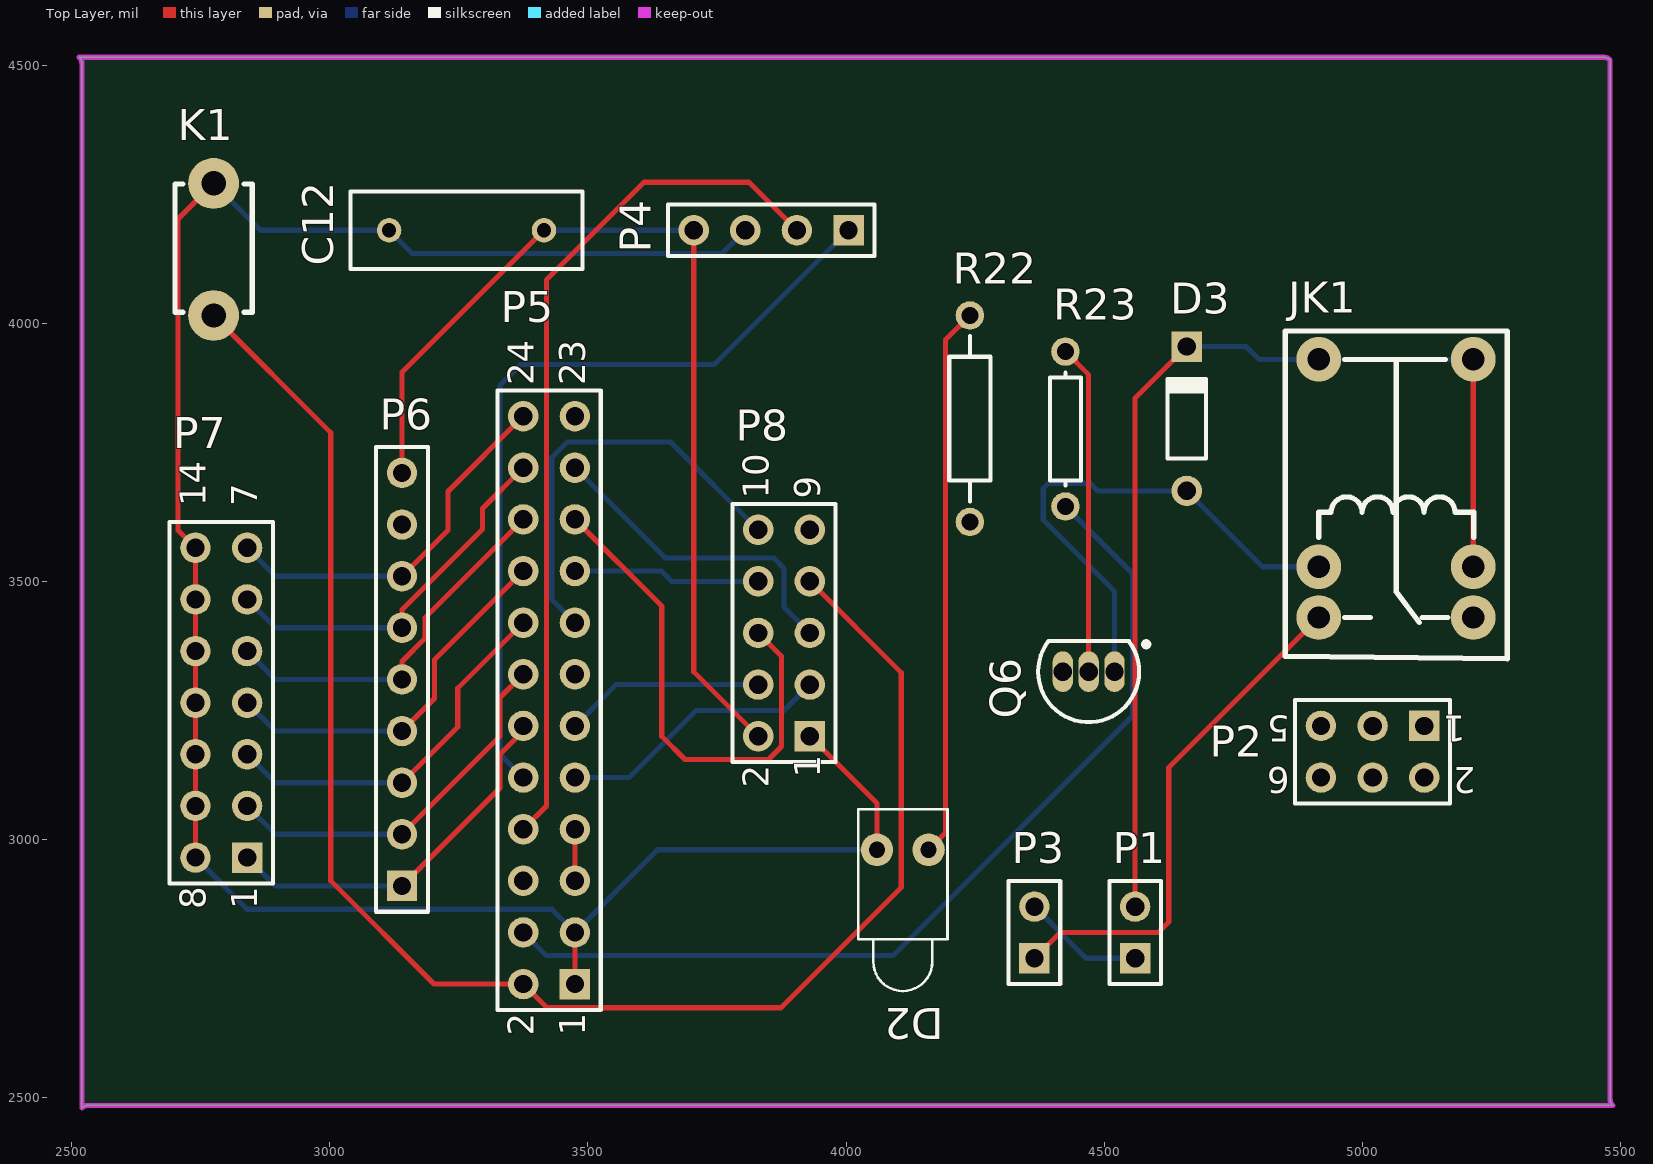
[diagram p0: Top Layer view]
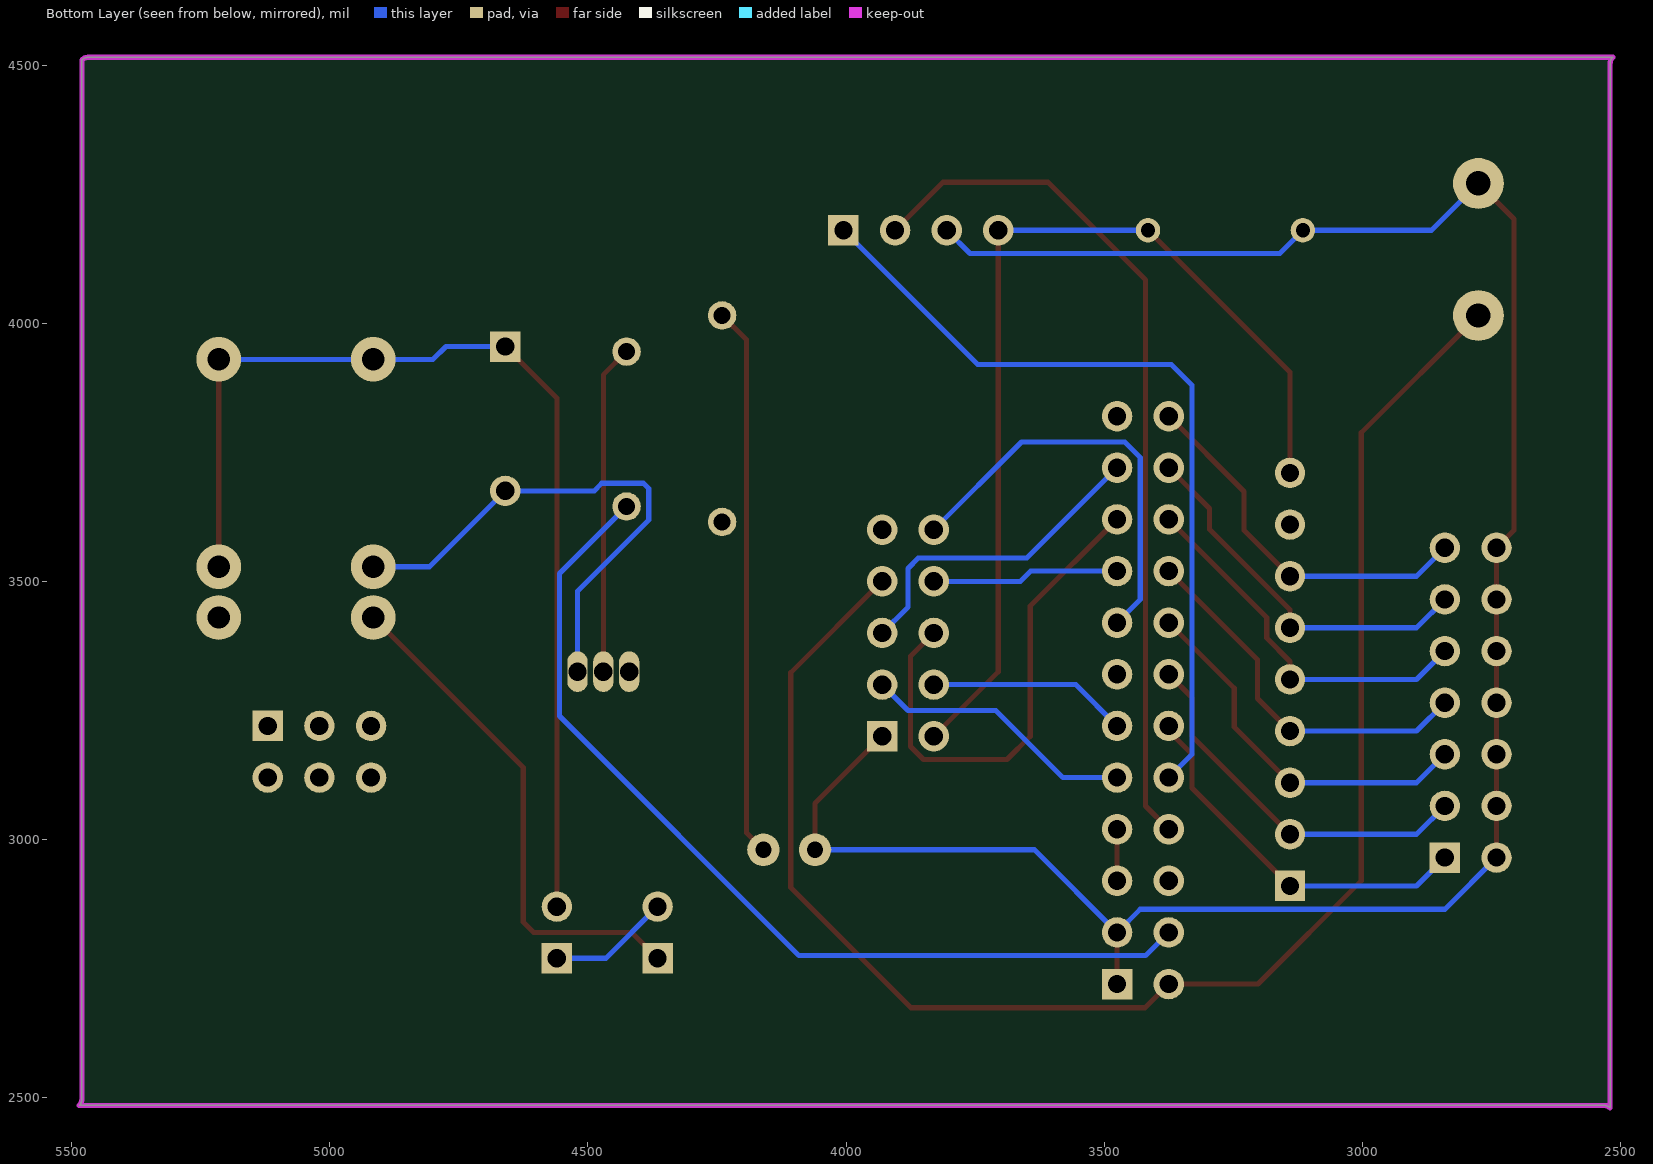
[diagram p1: Bottom Layer view, seen from below]
# Altium PCB MISC80684-5.PcbDoc
Units mil, origin at the board's own origin, x right, y up, seen from the top; angles counter-clockwise.
Board outline 2970 x 2035 mil, 2 copper layers (Top Layer, Bottom Layer); 16 components, 59 nets, 92 pads, 0 vias.

## Layer stack, top to bottom (the 12.6 mil dielectric is the usual default, probably not edited)
Top Solder: solder mask 0.4, Solder Resist, Dk 3.5
Top Layer: signal copper 1.4
Dielectric 1: dielectric 12.6, FR-4, Dk 4.8
Bottom Layer: signal copper 1.4
Bottom Solder: solder mask 0.4, Solder Resist, Dk 3.5

## Board outline
2520,2480 cw(c2532.07,2467.93) 2532.07,2485 5485,2485 cw(c5497.07,2497.07) 5480,2497.07 5480,4510 ccw(c5467.93,4497.93) 5467.93,4515 2515,4515 cw(c2502.93,4502.93) 2520,4502.93

## Design rules (kind name [scope] priority, off if disabled: settings)
Clearance [All] p1: gap=10
PolygonConnect [All] p1: connectstyle=Relief reliefconductorwidth=10 reliefentries=4 polygonreliefangle="90 Angle" airgapwidth=10
RoutingVias [All] p1: holewidth=28 width=50 viastyle="Through Hole" minholewidth=28 minwidth=50 maxholewidth=28 maxwidth=50
SolderMaskExpansion [All] p1: expansion=4
Width [All] p1: maxlimit=10 minlimit=10 preferedwidth=10
30 further rules are at their usual default settings.

## Components (designator, comment, footprint, x,y, rotation, side; value= is the part's Value field where it differs from the comment)
C12 "Cap" RAD-0.3 3265,4180 r180 top
D2 "LED1" LED-1 4110,2980 r270 top
D3 "Diode 1N914" DO-35 4660,3815 r90 top
JK1 "HRS1H-S-DC5V" HRS1H 4915.79,3930 r90 top
K1 "KEY" DIP-3X6X4.3 2775,4015 r90 top
P1 "Header 2" HDR1X2 4560,2770 r90 top
P2 "220V-5V-3.3V" HDR2X3 5120,3220 r180 top
P3 "Header 2" HDR1X2 4365,2770 r90 top
P4 "Header 4" HDR1X4 4005,4180 r180 top
P5 "Header 12X2" HDR2X12 3475,2720 r90 top
P6 "Header 9" HDR1X9 3140,2910 r90 top
P7 "Header 7X2A" HDR2X7_CEN 2840,2965 r90 top
P8 "Header 5X2" HDR2X5 3930,3200 r90 top
Q6 "2N3906" TO-92A 4470,3325 r90 top
R22 "Res2" AXIAL-0.4 4240,3815 r90 top
R23 "Res1" AXIAL-0.3 4425,3795 r90 top

## Footprints (in the part's own frame and the unit in brackets; to place one, negate y for a bottom-side part, rotate by r counter-clockwise, add the part's x,y. Pads: shape width x height; smd on the part's side, far side on the other; paste and mask are expansions set on the pad)
AXIAL-0.3 [mm] "Axial Device, Thru-Hole; 2 Leads; 0.3 in Pin Spacing"
  round 1.4 hole 0.85: 1(-3.81,0) 2(3.81,0)
  silkscreen extent -2.77,-0.76 2.77,0.76
AXIAL-0.4 [mm] "Axial Device, Thru-Hole; 2 Leads; 0.4 in Pin Spacing"
  round 1.4 hole 0.85: 1(-5.08,0) 2(5.08,0)
  silkscreen extent -4.06,-1.02 4.06,1.02
DIP-3X6X4.3 [mm]
  round 2.5 hole 1.2: 1(0,0) 3(6.5,0)
  silkscreen extent 0.16,-1.9 6.46,1.9, body extent -0.64,-1.75 7.19,1.75, height 4.31
DO-35 [mm] "Diode, Axial; Body 3.8 x 1.9 mm (LxDia. max), Lead Dia. 0.53 mm (max)"
  round 1.5 hole 0.9: 1(-3.55,0)
  rect 1.5x1.5 hole 0.9: 2(3.55,0)
  silkscreen extent -1.95,-0.95 2.05,0.95
HDR1X2 [mm] "Connector; Header; 2 Position"
  rect 1.5x1.5 hole 0.9: 1(0,0)
  round 1.5 hole 0.9: 2(2.54,0)
  silkscreen extent -1.27,-1.27 3.81,1.27
HDR1X4 [mm] "Connector; Header; 4 Position"
  rect 1.5x1.5 hole 0.9: 1(0,0)
  round 1.5 hole 0.9: 2(2.54,0) 3(5.08,0) 4(7.62,0)
  silkscreen extent -1.27,-1.27 8.89,1.27
HDR1X9 [mm] "Connector; Header; 9 Position"
  rect 1.5x1.5 hole 0.9: 1(0,0)
  round 1.5 hole 0.9: 2(2.54,0) 3(5.08,0) 4(7.62,0) 5(10.16,0) 6(12.7,0) 7(15.24,0) 8(17.78,0) 9(20.32,0)
  silkscreen extent -1.27,-1.27 21.59,1.27
HDR2X3 [mm] "Connector; Header; 3x2 Position"
  rect 1.5x1.5 hole 0.9: 1(0,0)
  round 1.5 hole 0.9: 2(0,2.54) 3(2.54,0) 4(2.54,2.54) 5(5.08,0) 6(5.08,2.54)
  silkscreen extent -1.27,-1.27 6.35,3.81
HDR2X5 [mm] "Connector; Header; 5x2 Position"
  rect 1.5x1.5 hole 0.9: 1(0,0)
  round 1.5 hole 0.9: 2(0,2.54) 3(2.54,0) 4(2.54,2.54) 5(5.08,0) 6(5.08,2.54) 7(7.62,0) 8(7.62,2.54) 9(10.16,0) 10(10.16,2.54)
  silkscreen extent -1.27,-1.27 11.43,3.81
HDR2X7_CEN [mm] "Connector; Header; 7x2 Position"
  rect 1.5x1.5 hole 0.9: 1(0,0)
  round 1.5 hole 0.9: 2(2.54,0) 3(5.08,0) 4(7.62,0) 5(10.16,0) 6(12.7,0) 7(15.24,0) 8(0,2.54) 9(2.54,2.54) 10(5.08,2.54) 11(7.62,2.54) 12(10.16,2.54) 13(12.7,2.54) 14(15.24,2.54)
  silkscreen extent -1.27,-1.27 16.51,3.81
HDR2X12 [mm] "Connector; Header; 12x2 Position"
  rect 1.5x1.5 hole 0.9: 1(0,0)
  round 1.5 hole 0.9: 2(0,2.54) 3(2.54,0) 4(2.54,2.54) 5(5.08,0) 6(5.08,2.54) 7(7.62,0) 8(7.62,2.54) 9(10.16,0) 10(10.16,2.54) 11(12.7,0) 12(12.7,2.54) 13(15.24,0) 14(15.24,2.54) 15(17.78,0) 16(17.78,2.54) 17(20.32,0) 18(20.32,2.54) 19(22.86,0) 20(22.86,2.54) 21(25.4,0) 22(25.4,2.54) 23(27.94,0) 24(27.94,2.54)
  silkscreen extent -1.27,-1.27 29.21,3.81
HRS1H [mm] "单刀双投"
  round 2.2 hole 1.1: 1(-10.2,0) 2(-10.2,-7.6) 3(0,0) 3(0,-7.6) 4(-12.7,0) 5(-12.7,-7.6)
  silkscreen extent -14.73,-9.27 1.4,1.65, body extent -14.35,-8.93 1.15,1.57, height 11.8
LED-1 [mm] "LED; 2 Leads"
  round 1.6 hole 0.8: 1(0,1.27) 2(0,-1.27)
  silkscreen extent -2,-2.2 6.95,2.2
RAD-0.3 [mm] "Radial Cap, Thru-Hole; 2 Leads; 0.3 in Pin Spacing"
  round 1.2 hole 0.7: 1(-3.81,0) 2(3.81,0)
  silkscreen extent -5.71,-1.91 5.71,1.91
TO-92A [mm] "TO, Flat Index; 3 In-Line, Axial Leads; Body Dia. 4.5mm; Leads 0.51 x 0.48 mm (max)"
  oval 2x1 hole 0.9: 1(0,-1.27) 2(0,0) 3(0,1.27)
  silkscreen extent -2.48,-2.96 1.5,2.48, body extent -2.48,-2.5 1.5,2.5, height 6.86

## Part data
C12: "Capacitor"
D2: "Typical RED GaAs LED"
D3: "High Conductance Fast Diode"
JK1: "5V一组转换"
P1 P3: "Header, 2-Pin"
P2: library part "Header 3X2", "Header, 3-Pin, Dual row"
P4: "Header, 4-Pin"
P5: "Header, 12-Pin, Dual row"
P6: "Header, 9-Pin"
P7: "Header, 7-Pin, Dual row"
P8: "Header, 5-Pin, Dual row"
Q6: "PNP General Purpose Amplifier"
R22 R23: "Resistor"

## Nets (pads, with @x,y where several pads share a name; then routed paths per layer and width w, separated by ;. In a path a pad name is that pad's centre, name@x,y a point inside that pad or via, vN(x,y) a via of type N, cw(c..) or ccw(c..) an arc to the next point about the centre after c; other vN are vias at no path point)
3.3: 
+12: 
GND: C12.2 D2.2 K1.3 P4.3 P5.1 P5.3 P7.8 P7.9 P7.10 P7.11 P7.12 P7.13 P7.14 P8.1 | length 4273.7
  Top Layer w10: P7.8 P7.9 P7.10 P7.11 P7.12 P7.13 P7.14 2706,3599 2706,4201.91 K1.3 ; P5.1 P5.3 ; P8.1 4060,3070 D2.2
  Bottom Layer w10: P7.8 2840,2865 3430,2865 P5.3 3635,2980 D2.2 ; K1.3 2865.91,4180 C12.2 3160,4135 3760,4135 P4.3
L: D3.2 JK1.2 JK1.3 P1.2 | length 2093
  Top Layer w10: P1.2 4560,3854.76 D3.2 ; JK1.2 JK1.3@5215,3930
  Bottom Layer w10: D3.2 4775,3954.76 4799.76,3930 4915.79,3930 JK1.3@5215,3930
N: P1.1 P3.2 | length 236.4
  Bottom Layer w10: P3.2 4465,2770 P1.1
NetC1_1: 
NetC2_1: 
NetC3_1: 
NetC3_2: 
NetC4_1: 
NetC5_1: 
NetC5_2: 
NetC6_2: 
NetC7_2: 
NetC8_1: 
NetC9_2: 
NetC10_1: 
NetC10_2: 
NetC11_1: 
NetC11_2: 
NetD1_1: 
NetD1_2: 
NetD2_1: D2.1 R22.2 | length 1068.1
  Top Layer w10: D2.1 4193,3013 4193,3968 R22.2
NetD3_1: D3.1 JK1.1 Q6.1 | length 1017
  Bottom Layer w10: Q6.1 4520,3481 4382,3619 4382,3680 4392,3690 4473,3690 4487.76,3675.24 D3.1 4806.81,3528.43 JK1.1
NetJK1_4: JK1.4 P3.1 | length 999.4
  Top Layer w10: P3.1 4415,2820 4605,2820 4625,2840 4625,3139.21 JK1.4
NetQ1_1: 
NetQ2_2: 
NetQ3_3: 
NetQ5_1: 
NetQ6_2: Q6.2 R23.2 | length 638.6
  Top Layer w10: R23.2 4470,3900 Q6.2
NetR6_2: 
NetR8_3: 
NetR19_1: 
NetR20_2: 
NetR21_1: 
P0.0: P5.4 R23.1 | length 1850.7
  Bottom Layer w10: P5.4 3420,2775 4091,2775 4555,3239 4555,3515 R23.1
P0.1: P5.6
P0.2: P4.2 P5.8 | length 1684.4
  Top Layer w10: P5.8 3420,3065 3420,4084 3609,4273 3812,4273 P4.2
P0.3: P4.1 P5.10 | length 1577.9
  Bottom Layer w10: P5.10 3330,3165 3330,3880 3370,3920 3745,3920 P4.1
P0.4: P5.12 P6.1 P7.1 | length 730.1
  Top Layer w10: P6.1 3330,3100 3330,3165 3375,3210 P5.12
  Bottom Layer w10: P7.1 2895,2910 P6.1
P0.5: P5.14 P6.2 P7.2 | length 730.1
  Top Layer w10: P6.2 3330,3200 3330,3275 P5.14
  Bottom Layer w10: P7.2 2895,3010 P6.2
P0.6: P5.16 P6.3 P7.3 | length 730.1
  Top Layer w10: P6.3 3248,3218 3248,3293 P5.16
  Bottom Layer w10: P7.3 2895,3110 P6.3
P0.7: P5.18 P6.4 P7.4 | length 730.1
  Top Layer w10: P6.4 3203,3273 3203,3348 P5.18
  Bottom Layer w10: P7.4 2895,3210 P6.4
P1.0: P5.20 P6.5 P7.5 | length 730.1
  Top Layer w10: P6.5 3140,3345 3185,3390 3185,3430 P5.20
  Bottom Layer w10: P7.5 2895,3310 P6.5
P1.1: P5.22 P6.6 P7.6 | length 730.1
  Top Layer w10: P6.6 3140,3445 3296,3601 3296,3641 P5.22
  Bottom Layer w10: P7.6 2895,3410 P6.6
P1.2: P5.24 P6.7 P7.7 | length 730.1
  Top Layer w10: P6.7 3229,3599 3229,3674 P5.24
  Bottom Layer w10: P7.7 2895,3510 P6.7
P1.3: P5.23
P1.4: P5.21 P8.5 | length 631.5
  Bottom Layer w10: P5.21 3650,3545 3860,3545 3880,3525 3880,3450 P8.5
P1.5: P5.19 P8.6 | length 989.2
  Top Layer w10: P5.19 3643,3452 3643,3200 3688,3155 3850,3155 3875,3180 3875,3355 P8.6
P1.6: P5.17 P8.8 | length 363.3
  Bottom Layer w10: P5.17 3642,3520 3662,3500 P8.8
P1.7: P5.15 P8.10 | length 821.5
  Bottom Layer w10: P5.15 3430,3465 3430,3740 3460,3770 3660,3770 P8.10
P2.0: P5.13
P2.1: P5.11 P8.4 | length 388.1
  Bottom Layer w10: P5.11 3555,3300 P8.4
P2.2: P5.9 P8.3 | length 529.6
  Bottom Layer w10: P5.9 3580,3120 3710,3250 3880,3250 P8.3
RESET: K1.1 P5.2 P8.7 | length 3158.8
  Top Layer w10: K1.1 3002,3788 3002,2920 3202,2720 P5.2 3421,2674 3874,2674 4107,2907 4107,3323 P8.7
VCC: R22.1
VCC3.3: C12.1 P4.4 P6.9 P8.2 | length 1905.7
  Top Layer w10: P6.9 3140,3905 C12.1 ; P4.4 3705,3325 P8.2
  Bottom Layer w10: C12.1 P4.4
VCC3.3V: P5.5 P5.7 | length 100
  Top Layer w10: P5.5 P5.7
VOUT: 
pads on no net: JK1.5 P2.1 P2.2 P2.3 P2.4 P2.5 P2.6 P6.8 P8.9 Q6.3

## Keep-outs
Keep-Out Layer:
  the board outline again, w10